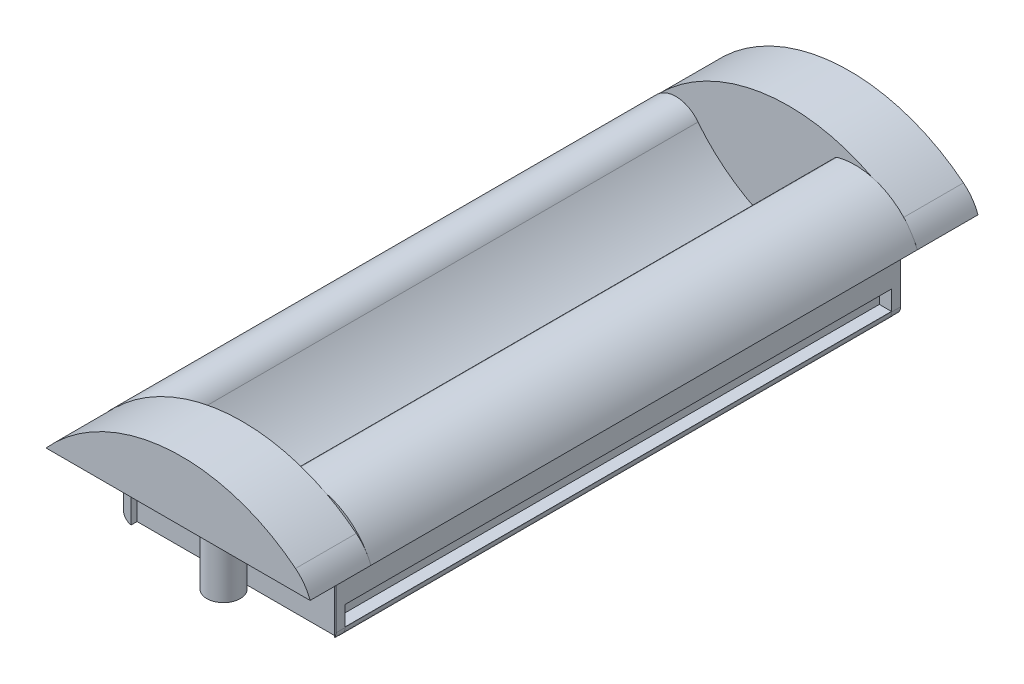
SolidWorks part; units mm, degrees
ref_plane "前视基准面" through (0, 0, 0) normal (0, 0, 1) x (1, 0, 0)
ref_plane "上视基准面" through (0, 0, 0) normal (0, 1, 0) x (1, 0, 0)
ref_plane "右视基准面" through (0, 0, 0) normal (1, 0, 0) x (0, 0, -1)
sketch "草图1" plane through (0, 0, 0) normal (0, 0, 1) x (1, 0, 0)
  line L0 (-15.5, 0) -> (15.5, 0)
  line L1 (0, 80.4208) -> (0, -78.8914) construction
  line L2 (-17, 1.5) -> (-17, 1.6)
  line L3 (-17, 1.6) -> (-15, 1.6)
  line L4 (-15, 1.6) -> (-15, 4.8)
  line L5 (-15, 4.8) -> (-18, 4.8)
  line L6 (-18, 4.8) -> (-18, 12.5)
  line L7 (-18, 12.5) -> (-22.25, 12.5)
  line L8 (21.25, 12.5) -> (17, 12.5)
  line L9 (17, 12.5) -> (17, 4.8)
  line L10 (17, 4.8) -> (15, 4.8)
  line L11 (15, 4.8) -> (15, 1.6)
  line L12 (15, 1.6) -> (17, 1.6)
  line L13 (17, 1.6) -> (17, 1.5)
  arc A0 (-15.5, 0) -> (-17, 1.5) centre (-15.5, 1.5) cw
  arc A1 (-22.25, 12.5) -> (-14.8721, 12.675) centre (-18.5, 10.0125) cw
  arc A2 (-14.8721, 12.675) -> (5.1279, 2.2193) centre (7, 30.1567) ccw
  arc A3 (5.1279, 2.2193) -> (15.7919, 12.5) centre (5.7965, 12.197) ccw
  arc A4 (15.7919, 12.5) -> (8.2692, 18.121) centre (9.7946, 12.3182) ccw
  arc A5 (8.2692, 18.121) -> (8.0058, 19.0857) centre (8.142, 18.6046) cw
  arc A6 (8.0058, 19.0857) -> (21.25, 12.5) centre (11.0024, 8.5017) cw
  arc A7 (15.5, 0) -> (17, 1.5) centre (15.5, 1.5) ccw
  point P11 (-17, 0)
  point P33 (17, 0)
  dimension "D3" = 1.5
  dimension "D11" = 6
  dimension "D15" = 1.5
  dimension "D18" = 4.5
  dimension "D19" = 28
  dimension "D20" = 0.5
  dimension "D21" = 11
  dimension "D26" = 8.142
  dimension "D10" = 10
  dimension "D1" = 17
  dimension "D2" = 17
  dimension "D4" = 2
  dimension "D5" = 3.2
  dimension "D6" = 12.5
  dimension "D7" = 4.25
  dimension "D8" = 1.6
  dimension "D9" = 20
  dimension "D12" = 12.5
  dimension "D13" = 3.2
  dimension "D14" = 1.6
  dimension "D16" = 2
  dimension "D17" = 18
  dimension "D22" = 4.25
  dimension "D23" = 18.5
  dimension "D24" = 7
extrude "凸台-拉伸1" add sketch "草图1" along normal mid plane 90
sketch "草图2" plane through (0, 0, 45) normal (0, 0, 1) x (1, 0, 0)
  line L0 (-22.25, 12.5) -> (-18, 12.5)
  line L1 (-18, 12.5) -> (-18, 1.5)
  line L2 (-16.5, 0) -> (16.5, 0)
  line L3 (17, 1.5) -> (17, 12.5)
  line L4 (17, 12.5) -> (21.25, 12.5)
  line L5 (17, 1.5) -> (17, 0)
  line L6 (17, 0) -> (16.5, 0)
  line L7 (-18, 1.5) -> (-18, 0)
  line L8 (-18, 0) -> (-16.5, 0)
  arc A0 (21.25, 12.5) -> (18.8537, 15.8644) centre (14.1159, 9.9543) ccw
  arc A1 (-22.25, 12.5) -> (18.8537, 15.8644) centre (0.0809, -7.553) cw
extrude "凸台-拉伸2" add sketch "草图2" along normal blind 10
mirror "镜向1" about plane through (0, 0, 0) normal (0, 0, 1) of "凸台-拉伸2"
sketch "草图3" plane through (0, 0, 0) normal (0, -1, 0) x (1, 0, 0)
  line L0 (0, 77.7797) -> (0, -82.3743) construction
  line L1 (-46.3834, 0) -> (66.2932, 0) construction
  line L2 (-46.3414, 50.55) -> (66.3353, 50.55) construction
  line L3 (1.1456, 45.5) -> (16.73, 45.5)
  line L4 (-16.73, 46.5) -> (-16.73, 45.5)
  line L5 (-16.73, 45.5) -> (-1.1456, 45.5)
  line L6 (-18, 46.5) -> (-18, 55)
  line L7 (-18, 55) -> (18, 55)
  line L8 (18, 46.5) -> (18, 55)
  line L9 (-18, 46.1) -> (18, 55) construction
  line L10 (-18, 55) -> (18, 46.1) construction
  line L11 (16.73, 46.5) -> (18, 46.5)
  line L12 (16.73, 46.5) -> (16.73, 45.5)
  line L13 (-18, -46.5) -> (-18, -55)
  line L14 (-18, -55) -> (18, -55)
  line L15 (16.73, 46.5) -> (18, 46.1) construction
  line L16 (16.73, 45.5) -> (18, 46.5) construction
  line L17 (-16.73, 46.5) -> (-18, 46.5)
  line L18 (-16.73, 46.5) -> (-18, 46.1) construction
  line L19 (-16.73, 45.5) -> (-18, 46.5) construction
  line L20 (18, -46.5) -> (18, -55)
  line L21 (16.73, -46.5) -> (18, -46.5)
  line L22 (16.73, -46.5) -> (16.73, -45.5)
  line L23 (1.1456, -45.5) -> (16.73, -45.5)
  line L24 (-16.73, -45.5) -> (-1.1456, -45.5)
  line L25 (-16.73, -46.5) -> (-18, -46.5)
  line L26 (-16.73, -46.5) -> (-16.73, -45.5)
  line L28 (-22.25, -55) -> (-18, -55) construction
  circle A0 centre (0, 50.55) radius 4.3449 construction
  arc A1 (1.1456, 45.5) -> (-1.1456, 45.5) centre (0, 48) ccw
  arc A2 (1.1456, -45.5) -> (-1.1456, -45.5) centre (0, -48) cw
  point P18 (17.6371, 46.2143)
  point P25 (-17.6371, 46.2143)
  dimension "D2" = 5.5
  dimension "D1" = 4.45
  dimension "D3" = 1.27
  dimension "D4" = 1
  dimension "D5" = 2.5
  dimension "D6" = 36
  dimension "D7" = 96
extrude "切除-拉伸11" cut sketch "草图3" against normal blind 12.5
fillet "圆角1" radius 1.5 4 edges at (-18, 0, -45.75) (17, 0, -45.75) (17, 0, 45.75) (-18, 0, 45.75)
sketch "草图4" plane through (0, 0, 0) normal (0, -1, 0) x (1, 0, 0)
  circle A0 centre (0, 48) radius 1.7
  circle A1 centre (0, -48) radius 1.7
extrude "切除-拉伸12" cut sketch "草图4" against normal blind 11.25
